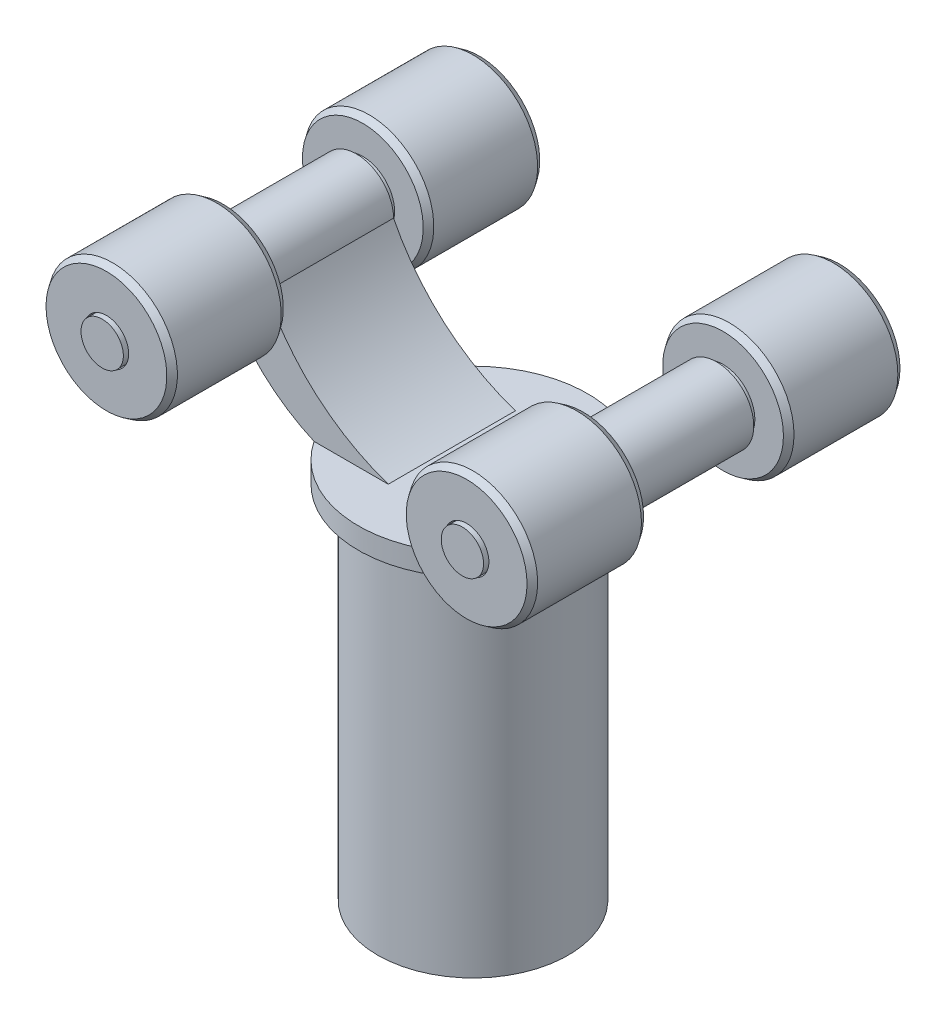
from build123d import *

# Parameters (mm, degrees)
SKETCH1_R                  = 45
BOSS_EXTRUDE1_DEPTH        = 180
BOSS_EXTRUDE2_DEPTH        = 90
BOSS_EXTRUDE2_DEPTH_BACK   = 90
SKETCH3_R                  = 10
BOSS_EXTRUDE2_2_DEPTH      = 90
BOSS_EXTRUDE2_2_DEPTH_BACK = 90
BOSS_EXTRUDE3_DEPTH        = 30
BOSS_EXTRUDE3_DEPTH_BACK   = 30
SKETCH5_R                  = 54.083269132
BOSS_EXTRUDE4_DEPTH        = 10
SKETCH6_R                  = 15
BOSS_EXTRUDE5_DEPTH        = 3
BOSS_EXTRUDE6_START        = 3
SKETCH7_R                  = 15
BOSS_EXTRUDE6_DEPTH        = 3


with BuildPart() as part:
    # Sketch1 → Boss-Extrude1 (new body)
    with BuildSketch(Plane(origin=(0, 0, 0), x_dir=(1, 0, 0), z_dir=(0, 1, 0))):
        with Locations(Location((0, 0, 0), (0, 0, 90))):
            Circle(SKETCH1_R)
    extrude(amount=BOSS_EXTRUDE1_DEPTH)



with BuildPart() as body_2:
    # Sketch3 → Boss-Extrude2 (new, two sides: drawn at the far end of the back side and taken through both)
    with BuildSketch(Plane.XY.offset(-BOSS_EXTRUDE2_DEPTH_BACK)):
        with Locations((85, 230)):
            Circle(SKETCH3_R)
    extrude(amount=BOSS_EXTRUDE2_DEPTH + BOSS_EXTRUDE2_DEPTH_BACK)


with BuildPart() as body_3:
    # Sketch3 → Boss-Extrude2 2 (new, two sides: drawn at the far end of the back side and taken through both)
    with BuildSketch(Plane.XY.offset(-BOSS_EXTRUDE2_2_DEPTH_BACK)):
        with Locations((-85, 230)):
            Circle(SKETCH3_R)
    extrude(amount=BOSS_EXTRUDE2_2_DEPTH + BOSS_EXTRUDE2_2_DEPTH_BACK)


with BuildPart() as part_1:
    add(part.part)

    add(body_2.part)  # Boss-Extrude3 merges body 2

    add(body_3.part)  # Boss-Extrude3 merges body 3
    # Sketch4 → Boss-Extrude3 (add, two sides: drawn at the far end of the back side and taken through both)
    with BuildSketch(Plane.XY.offset(-BOSS_EXTRUDE3_DEPTH_BACK)):
        with BuildLine():
            Line((-45, 180), (-10, 180))
            ThreePointArc((-10, 180), (-43.69905694, 199.308584519), (-67.5, 230))
            ThreePointArc((-67.5, 230), (-98.082305532, 241.623393737), (-82.940375083, 212.621624207))
            ThreePointArc((-82.940375083, 212.621624207), (-66.424952125, 193.455813577), (-45, 180))
        make_face()
        with BuildLine():
            Line((10, 180), (45, 180))
            ThreePointArc((45, 180), (60.253550288, 202.66599047), (67.528581994, 229.00022359))
            ThreePointArc((67.528581994, 229.00022359), (102.492853042, 230.500092441), (67.5, 230))
            ThreePointArc((67.5, 230), (43.69905694, 199.308584519), (10, 180))
        make_face()
    extrude(amount=BOSS_EXTRUDE3_DEPTH + BOSS_EXTRUDE3_DEPTH_BACK)

    # Sketch5 → Boss-Extrude4 (add)
    with BuildSketch(Plane.XZ.offset(-180)):
        with Locations(Location((0, 0, 0), (0, 0, 33.690067526))):
            Circle(SKETCH5_R)
    extrude(amount=BOSS_EXTRUDE4_DEPTH)

    # Sketch6 → Boss-Extrude5 (add)
    with BuildSketch(Plane.XY.offset(30)):
        with Locations((-85, 230)):
            Circle(SKETCH6_R)
        with Locations(Location((85, 230, 0), (0, 0, 180))):
            Circle(SKETCH6_R)
    extrude(amount=BOSS_EXTRUDE5_DEPTH)

    # Sketch7 → Boss-Extrude6 (add)
    with BuildSketch(Plane(origin=(0, 0, -30), x_dir=(-1, 0, 0), z_dir=(0, 0, -1)).offset(BOSS_EXTRUDE6_START)):
        with Locations((-85, 230)):
            Circle(SKETCH7_R)
        with Locations(Location((85, 230, 0), (0, 0, 180))):
            Circle(SKETCH7_R)
    extrude(amount=-BOSS_EXTRUDE6_DEPTH)

    # Sketch8 → Revolve1 (revolve)
    with BuildSketch(Plane(origin=(-85, 0, 0), x_dir=(0, 0, -1), z_dir=(1, 0, 0)), mode=Mode.PRIVATE) as revolve1_sk:
        Polygon((-33, 240.5), (-33, 258.5), (-36, 260.5), (-85, 260.5), (-88, 258.5), (-88, 240.5), align=None)
    revolve1 = revolve(revolve1_sk.sketch.rotate(Axis((-85, 230, 33), (0, 0, 1)), 90), axis=Axis((-85, 230, 33), (0, 0, 1)))

    # Mirror1: Revolve1 across plane
    add(revolve1.mirror(Plane(origin=(0, 0, 0), x_dir=(0, 0, 1), z_dir=(1, 0, 0))))

    # Mirror2: Revolve1 across plane
    add(revolve1.mirror(Plane.XY))

    # Mirror2 copy 1 sketch → Mirror2 copy 1 (revolve)
    with BuildSketch(Plane.ZY.offset(-85)):
        Polygon((-33, 240.5), (-33, 258.5), (-36, 260.5), (-85, 260.5), (-88, 258.5), (-88, 240.5), align=None)
    revolve(axis=Axis((85, 230, -33), (0, 0, -1)))


solid = part_1.part
